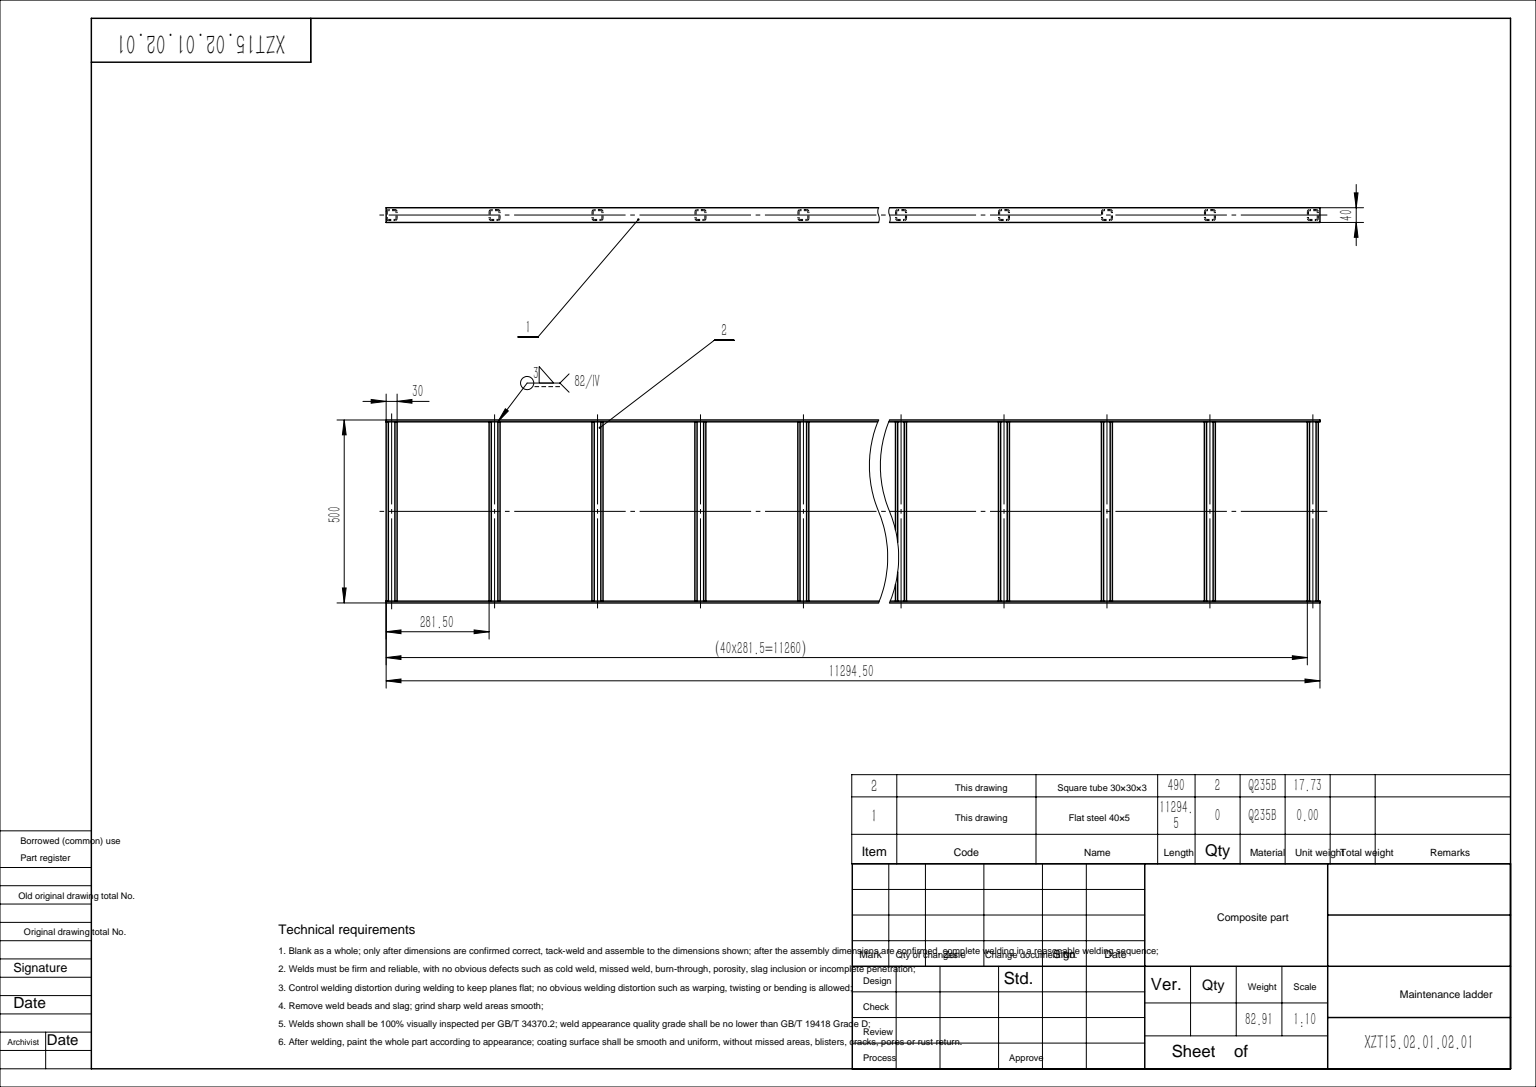
from build123d import *

# Parameters (mm, degrees)
SWEEP2_PROFILE_R                               = 6
CHAMFER1_SIZE                                  = 0.5
SKETCH14_W                                     = 40
SKETCH14_H                                     = 5
GB_T_704_1988_HOT_ROLLED_FLAT_STEEL_40_5_DEPTH = 11294.5
SKETCH14_ON_SEGMENT_2_W                        = 40
SKETCH14_ON_SEGMENT_2_H                        = 5
GB_T_704_1988_HOT_ROLLED_FLAT_STEEL_2_DEPTH    = 11294.5
GB_T_6728_2002_SQUARE_HOLLOW_SECTION_30_DEPTH  = 495
GB_T_6728_2002_SQUARE_HOLLOW_SECTION_2_DEPTH   = 495
LINEARPATTERN1_COUNT                           = 40
LINEARPATTERN1_PITCH                           = 281.5
CUT_EXTRUDE1_DEPTH                             = 11072.322187324
CUT_EXTRUDE1_DEPTH_BACK                        = 11072.322187324


with BuildPart() as part:
    # Sweep2: sweep along a path in 草图1
    with BuildLine(Plane.XY) as sweep2_path:
        Line((2.366140089, 179), (-19.767570176, 101.810579127))
        ThreePointArc((-19.767570176, 101.810579127), (-19.941608412, 100.991793598), (-20, 100.156754992))
        Line((-20, 100.156754992), (-20, 0))
        ThreePointArc((-20, 0), (14.142135624, -14.142135624), (0, 20))
        Line((0, 20), (-13.95, 20))
    # Sweep2 profile (on start of the path) → Sweep2 (sweep)
    with BuildSketch(Plane(origin=(2.366140089, 179, 0), x_dir=(-0.9612616959383187, 0.27563735581700005, 0), z_dir=(-0.27563735581700005, -0.9612616959383187, 0))):
        Circle(SWEEP2_PROFILE_R)
    sweep(path=sweep2_path.line)

    # Chamfer1
    chamfer1_edges = [part.edges().sort_by_distance(p)[0] for p in [
        (8.133710265, 177.346175865, 0),
    ]]
    chamfer(chamfer1_edges, length=CHAMFER1_SIZE)

    # Sketch10 → Cut-Extrude1 (cut, two sides: drawn at the far end of the back side and taken through both)
    with BuildSketch(Plane.XY.offset(20).offset(-CUT_EXTRUDE1_DEPTH_BACK)):
        Polygon((2.946393984, 202.791317487), (-74.47486017, -67.208682513), (40.52513983, -100.184401876), (117.946393984, 169.815598124), align=None)
    extrude(amount=CUT_EXTRUDE1_DEPTH + CUT_EXTRUDE1_DEPTH_BACK, mode=Mode.SUBTRACT)


with BuildPart() as body_2:
    # Sketch14 → GB/T 704-1988 hot-rolled flat steel 40×5(1) (new body)
    with BuildSketch(Plane(origin=(-3062.838260977, -10488.870369932, -20), x_dir=(0, 0, 1), z_dir=(-0.2756373558169933, -0.9612616959383206, 0))):
        with Locations((20, 2.5)):
            Rectangle(SKETCH14_W, SKETCH14_H)
    extrude(amount=-GB_T_704_1988_HOT_ROLLED_FLAT_STEEL_40_5_DEPTH)


with BuildPart() as body_3:
    # Sketch14 on segment 2 (carried to segment 2) → GB_T 704-1988 hot-rolled flat steel  2 (new body)
    with BuildSketch(Plane(origin=(-425.476685192, 504.540345972, -20), x_dir=(0, 0, 1), z_dir=(-0.275637356, -0.961261696, 0))):
        with Locations((20, 2.5)):
            Rectangle(SKETCH14_ON_SEGMENT_2_W, SKETCH14_ON_SEGMENT_2_H)
    extrude(amount=GB_T_704_1988_HOT_ROLLED_FLAT_STEEL_2_DEPTH)


with BuildPart() as body_4:
    # Sketch1 → GB/T 6728-2002 square hollow section 30×3-example.com(1) (new body)
    with BuildSketch(Plane(origin=(-3534.528240129, -10338.010953364, 0), x_dir=(0.2756373558170007, 0.9612616959383186, 0), z_dir=(0.9612616959383186, -0.2756373558170007, 0))):
        with BuildLine():
            Line((-9, -15), (9, -15))
            ThreePointArc((9, -15), (13.242640687, -13.242640687), (15, -9))
            Line((15, -9), (15, 9))
            ThreePointArc((15, 9), (13.242640687, 13.242640687), (9, 15))
            Line((9, 15), (-9, 15))
            ThreePointArc((-9, 15), (-13.242640687, 13.242640687), (-15, 9))
            Line((-15, 9), (-15, -9))
            ThreePointArc((-15, -9), (-13.242640687, -13.242640687), (-9, -15))
        make_face()
        with BuildLine():
            Line((-9, -12), (9, -12))
            ThreePointArc((9, -12), (11.121320344, -11.121320344), (12, -9))
            Line((12, -9), (12, 9))
            ThreePointArc((12, 9), (11.121320344, 11.121320344), (9, 12))
            Line((9, 12), (-9, 12))
            ThreePointArc((-9, 12), (-11.121320344, 11.121320344), (-12, 9))
            Line((-12, 9), (-12, -9))
            ThreePointArc((-12, -9), (-11.121320344, -11.121320344), (-9, -12))
        make_face(mode=Mode.SUBTRACT)
    extrude(amount=GB_T_6728_2002_SQUARE_HOLLOW_SECTION_30_DEPTH)

    # Trim_Extend1 15
    split(bisect_by=Plane(origin=(-55.815282461, 16.0047747, 0), x_dir=(-0.275637356, -0.961261696, 0), z_dir=(-0.961261696, 0.275637356, 0)), keep=Keep.TOP)


with BuildPart() as body_5:
    # Sketch1 on segment 2 (carried to segment 2) → GB_T 6728-2002 square hollow section 2 (new body)
    with BuildSketch(Plane(origin=(-3456.936324467, -10067.415785957, 0), x_dir=(0.275637356, 0.961261696, 0), z_dir=(0.961261696, -0.275637356, 0))):
        with BuildLine():
            Line((-9, -15), (9, -15))
            ThreePointArc((9, -15), (13.242640687, -13.242640687), (15, -9))
            Line((15, -9), (15, 9))
            ThreePointArc((15, 9), (13.242640687, 13.242640687), (9, 15))
            Line((9, 15), (-9, 15))
            ThreePointArc((-9, 15), (-13.242640687, 13.242640687), (-15, 9))
            Line((-15, 9), (-15, -9))
            ThreePointArc((-15, -9), (-13.242640687, -13.242640687), (-9, -15))
        make_face()
        with BuildLine():
            Line((-9, -12), (9, -12))
            ThreePointArc((9, -12), (11.121320344, -11.121320344), (12, -9))
            Line((12, -9), (12, 9))
            ThreePointArc((12, 9), (11.121320344, 11.121320344), (9, 12))
            Line((9, 12), (-9, 12))
            ThreePointArc((-9, 12), (-11.121320344, 11.121320344), (-12, 9))
            Line((-12, 9), (-12, -9))
            ThreePointArc((-12, -9), (-11.121320344, -11.121320344), (-9, -12))
        make_face(mode=Mode.SUBTRACT)
    extrude(amount=GB_T_6728_2002_SQUARE_HOLLOW_SECTION_2_DEPTH)

    # Trim_Extend1 15
    split(bisect_by=Plane(origin=(-55.815282461, 16.0047747, 0), x_dir=(-0.275637356, -0.961261696, 0), z_dir=(-0.961261696, 0.275637356, 0)), keep=Keep.TOP)


with BuildPart() as linearpattern1_1:
    # LinearPattern1: pattern copy
    add(body_5.part.moved(Location(Vector(0.2756373558170005, 0.9612616959383186, 0) * (1 * LINEARPATTERN1_PITCH))))


with BuildPart() as linearpattern1_2:
    # LinearPattern1: pattern copy
    add(body_5.part.moved(Location(Vector(0.2756373558170005, 0.9612616959383186, 0) * (2 * LINEARPATTERN1_PITCH))))


with BuildPart() as linearpattern1_3:
    # LinearPattern1: pattern copy
    add(body_5.part.moved(Location(Vector(0.2756373558170005, 0.9612616959383186, 0) * (3 * LINEARPATTERN1_PITCH))))


with BuildPart() as linearpattern1_4:
    # LinearPattern1: pattern copy
    add(body_5.part.moved(Location(Vector(0.2756373558170005, 0.9612616959383186, 0) * (4 * LINEARPATTERN1_PITCH))))


with BuildPart() as linearpattern1_5:
    # LinearPattern1: pattern copy
    add(body_5.part.moved(Location(Vector(0.2756373558170005, 0.9612616959383186, 0) * (5 * LINEARPATTERN1_PITCH))))


with BuildPart() as linearpattern1_6:
    # LinearPattern1: pattern copy
    add(body_5.part.moved(Location(Vector(0.2756373558170005, 0.9612616959383186, 0) * (6 * LINEARPATTERN1_PITCH))))


with BuildPart() as linearpattern1_7:
    # LinearPattern1: pattern copy
    add(body_5.part.moved(Location(Vector(0.2756373558170005, 0.9612616959383186, 0) * (7 * LINEARPATTERN1_PITCH))))


with BuildPart() as linearpattern1_8:
    # LinearPattern1: pattern copy
    add(body_5.part.moved(Location(Vector(0.2756373558170005, 0.9612616959383186, 0) * (8 * LINEARPATTERN1_PITCH))))


with BuildPart() as linearpattern1_9:
    # LinearPattern1: pattern copy
    add(body_5.part.moved(Location(Vector(0.2756373558170005, 0.9612616959383186, 0) * (9 * LINEARPATTERN1_PITCH))))


with BuildPart() as linearpattern1_10:
    # LinearPattern1: pattern copy
    add(body_5.part.moved(Location(Vector(0.2756373558170005, 0.9612616959383186, 0) * (10 * LINEARPATTERN1_PITCH))))


with BuildPart() as linearpattern1_11:
    # LinearPattern1: pattern copy
    add(body_5.part.moved(Location(Vector(0.2756373558170005, 0.9612616959383186, 0) * (11 * LINEARPATTERN1_PITCH))))


with BuildPart() as linearpattern1_12:
    # LinearPattern1: pattern copy
    add(body_5.part.moved(Location(Vector(0.2756373558170005, 0.9612616959383186, 0) * (12 * LINEARPATTERN1_PITCH))))


with BuildPart() as linearpattern1_13:
    # LinearPattern1: pattern copy
    add(body_5.part.moved(Location(Vector(0.2756373558170005, 0.9612616959383186, 0) * (13 * LINEARPATTERN1_PITCH))))


with BuildPart() as linearpattern1_14:
    # LinearPattern1: pattern copy
    add(body_5.part.moved(Location(Vector(0.2756373558170005, 0.9612616959383186, 0) * (14 * LINEARPATTERN1_PITCH))))


with BuildPart() as linearpattern1_15:
    # LinearPattern1: pattern copy
    add(body_5.part.moved(Location(Vector(0.2756373558170005, 0.9612616959383186, 0) * (15 * LINEARPATTERN1_PITCH))))


with BuildPart() as linearpattern1_16:
    # LinearPattern1: pattern copy
    add(body_5.part.moved(Location(Vector(0.2756373558170005, 0.9612616959383186, 0) * (16 * LINEARPATTERN1_PITCH))))


with BuildPart() as linearpattern1_17:
    # LinearPattern1: pattern copy
    add(body_5.part.moved(Location(Vector(0.2756373558170005, 0.9612616959383186, 0) * (17 * LINEARPATTERN1_PITCH))))


with BuildPart() as linearpattern1_18:
    # LinearPattern1: pattern copy
    add(body_5.part.moved(Location(Vector(0.2756373558170005, 0.9612616959383186, 0) * (18 * LINEARPATTERN1_PITCH))))


with BuildPart() as linearpattern1_19:
    # LinearPattern1: pattern copy
    add(body_5.part.moved(Location(Vector(0.2756373558170005, 0.9612616959383186, 0) * (19 * LINEARPATTERN1_PITCH))))


with BuildPart() as linearpattern1_20:
    # LinearPattern1: pattern copy
    add(body_5.part.moved(Location(Vector(0.2756373558170005, 0.9612616959383186, 0) * (20 * LINEARPATTERN1_PITCH))))


with BuildPart() as linearpattern1_21:
    # LinearPattern1: pattern copy
    add(body_5.part.moved(Location(Vector(0.2756373558170005, 0.9612616959383186, 0) * (21 * LINEARPATTERN1_PITCH))))


with BuildPart() as linearpattern1_22:
    # LinearPattern1: pattern copy
    add(body_5.part.moved(Location(Vector(0.2756373558170005, 0.9612616959383186, 0) * (22 * LINEARPATTERN1_PITCH))))


with BuildPart() as linearpattern1_23:
    # LinearPattern1: pattern copy
    add(body_5.part.moved(Location(Vector(0.2756373558170005, 0.9612616959383186, 0) * (23 * LINEARPATTERN1_PITCH))))


with BuildPart() as linearpattern1_24:
    # LinearPattern1: pattern copy
    add(body_5.part.moved(Location(Vector(0.2756373558170005, 0.9612616959383186, 0) * (24 * LINEARPATTERN1_PITCH))))


with BuildPart() as linearpattern1_25:
    # LinearPattern1: pattern copy
    add(body_5.part.moved(Location(Vector(0.2756373558170005, 0.9612616959383186, 0) * (25 * LINEARPATTERN1_PITCH))))


with BuildPart() as linearpattern1_26:
    # LinearPattern1: pattern copy
    add(body_5.part.moved(Location(Vector(0.2756373558170005, 0.9612616959383186, 0) * (26 * LINEARPATTERN1_PITCH))))


with BuildPart() as linearpattern1_27:
    # LinearPattern1: pattern copy
    add(body_5.part.moved(Location(Vector(0.2756373558170005, 0.9612616959383186, 0) * (27 * LINEARPATTERN1_PITCH))))


with BuildPart() as linearpattern1_28:
    # LinearPattern1: pattern copy
    add(body_5.part.moved(Location(Vector(0.2756373558170005, 0.9612616959383186, 0) * (28 * LINEARPATTERN1_PITCH))))


with BuildPart() as linearpattern1_29:
    # LinearPattern1: pattern copy
    add(body_5.part.moved(Location(Vector(0.2756373558170005, 0.9612616959383186, 0) * (29 * LINEARPATTERN1_PITCH))))


with BuildPart() as linearpattern1_30:
    # LinearPattern1: pattern copy
    add(body_5.part.moved(Location(Vector(0.2756373558170005, 0.9612616959383186, 0) * (30 * LINEARPATTERN1_PITCH))))


with BuildPart() as linearpattern1_31:
    # LinearPattern1: pattern copy
    add(body_5.part.moved(Location(Vector(0.2756373558170005, 0.9612616959383186, 0) * (31 * LINEARPATTERN1_PITCH))))


with BuildPart() as linearpattern1_32:
    # LinearPattern1: pattern copy
    add(body_5.part.moved(Location(Vector(0.2756373558170005, 0.9612616959383186, 0) * (32 * LINEARPATTERN1_PITCH))))


with BuildPart() as linearpattern1_33:
    # LinearPattern1: pattern copy
    add(body_5.part.moved(Location(Vector(0.2756373558170005, 0.9612616959383186, 0) * (33 * LINEARPATTERN1_PITCH))))


with BuildPart() as linearpattern1_34:
    # LinearPattern1: pattern copy
    add(body_5.part.moved(Location(Vector(0.2756373558170005, 0.9612616959383186, 0) * (34 * LINEARPATTERN1_PITCH))))


with BuildPart() as linearpattern1_35:
    # LinearPattern1: pattern copy
    add(body_5.part.moved(Location(Vector(0.2756373558170005, 0.9612616959383186, 0) * (35 * LINEARPATTERN1_PITCH))))


with BuildPart() as linearpattern1_36:
    # LinearPattern1: pattern copy
    add(body_5.part.moved(Location(Vector(0.2756373558170005, 0.9612616959383186, 0) * (36 * LINEARPATTERN1_PITCH))))


with BuildPart() as linearpattern1_37:
    # LinearPattern1: pattern copy
    add(body_5.part.moved(Location(Vector(0.2756373558170005, 0.9612616959383186, 0) * (37 * LINEARPATTERN1_PITCH))))


with BuildPart() as linearpattern1_38:
    # LinearPattern1: pattern copy
    add(body_5.part.moved(Location(Vector(0.2756373558170005, 0.9612616959383186, 0) * (38 * LINEARPATTERN1_PITCH))))


with BuildPart() as linearpattern1_39:
    # LinearPattern1: pattern copy
    add(body_5.part.moved(Location(Vector(0.2756373558170005, 0.9612616959383186, 0) * (39 * LINEARPATTERN1_PITCH))))


solid = Compound([body_2.part, body_3.part, body_4.part, body_5.part, linearpattern1_1.part, linearpattern1_2.part, linearpattern1_3.part, linearpattern1_4.part, linearpattern1_5.part, linearpattern1_6.part, linearpattern1_7.part, linearpattern1_8.part, linearpattern1_9.part, linearpattern1_10.part, linearpattern1_11.part, linearpattern1_12.part, linearpattern1_13.part, linearpattern1_14.part, linearpattern1_15.part, linearpattern1_16.part, linearpattern1_17.part, linearpattern1_18.part, linearpattern1_19.part, linearpattern1_20.part, linearpattern1_21.part, linearpattern1_22.part, linearpattern1_23.part, linearpattern1_24.part, linearpattern1_25.part, linearpattern1_26.part, linearpattern1_27.part, linearpattern1_28.part, linearpattern1_29.part, linearpattern1_30.part, linearpattern1_31.part, linearpattern1_32.part, linearpattern1_33.part, linearpattern1_34.part, linearpattern1_35.part, linearpattern1_36.part, linearpattern1_37.part, linearpattern1_38.part, linearpattern1_39.part])
